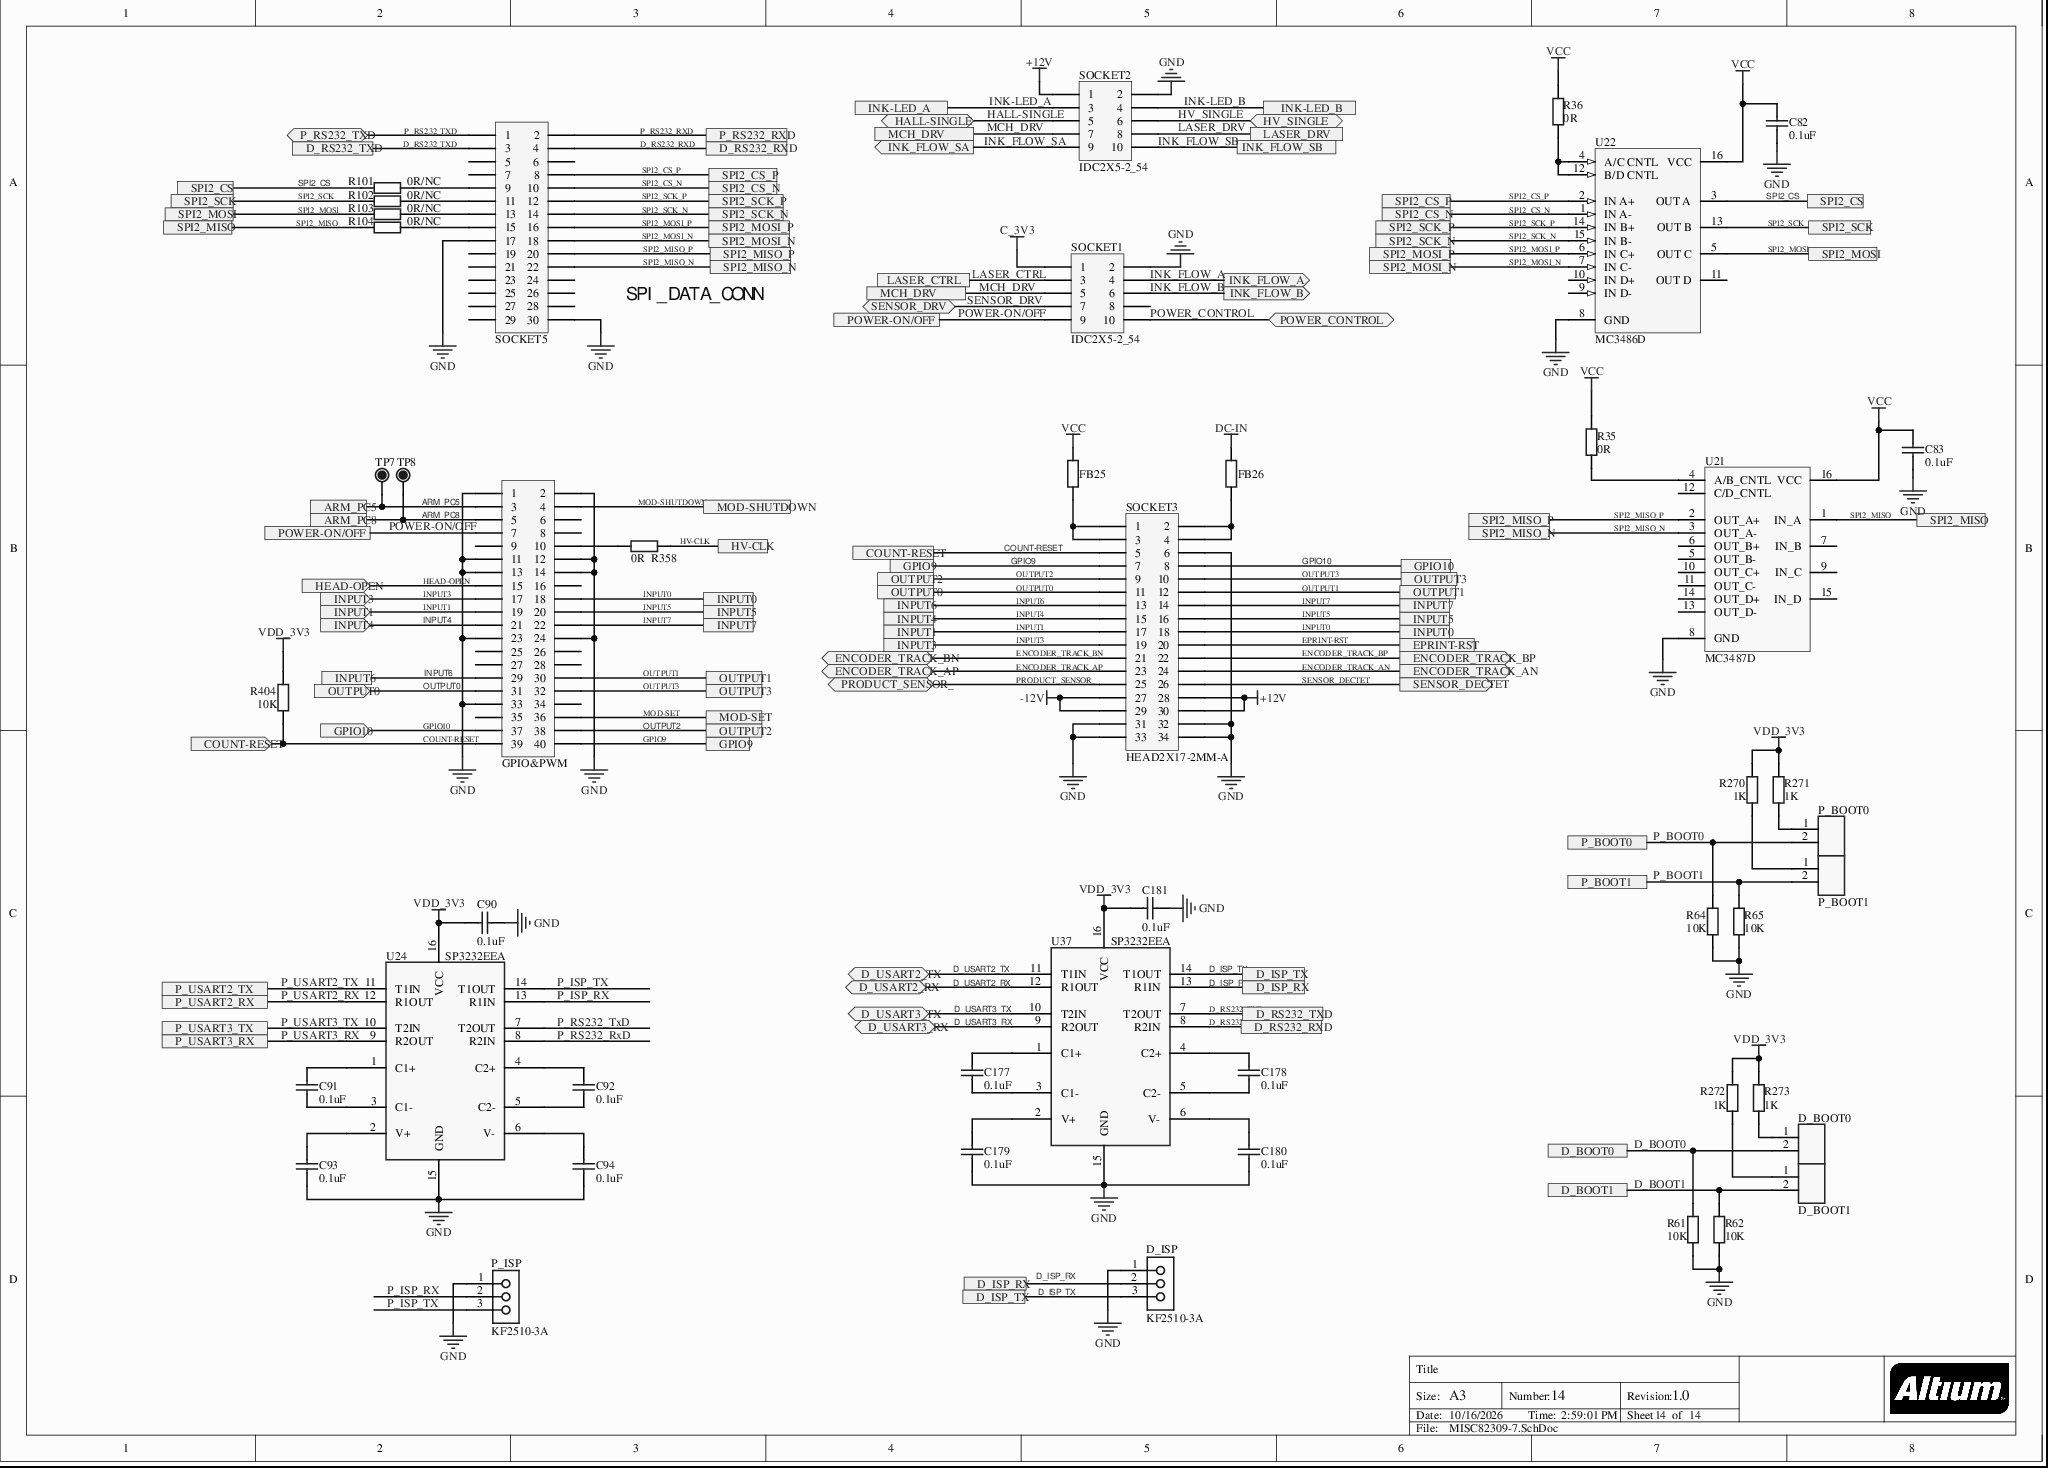
[diagram p0: MISC82309-7.SchDoc]
# Altium project MISC82309-16.PrjPcb (part 6 of 6)

## Sheet MISC82309-7.SchDoc
size A3; DocumentNumber: 14; Revision: 1.0; SheetNumber: 14; SheetTotal: 14

### Parts
C82  0.1uF  [CAP_0805]
C83  0.1uF  [CAP_0805]
C90  0.1uF  [C0603]
C91  0.1uF  [C0603]
C92  0.1uF  [C0603]
C93  0.1uF  [C0603]
C94  0.1uF  [C0603]
C177  0.1uF  [C0603]
C178  0.1uF  [C0603]
C179  0.1uF  [C0603]
C180  0.1uF  [C0603]
C181  0.1uF  [C0603]
D_BOOT0  PLS-2  [PLS-2-2_54]  (value not drawn)
D_BOOT1  PLS-2  [PLS-2-2_54]  (value not drawn)
D_ISP  KF2510-3A  [KF2510-3A]
FB25  60  [SMD1206-L]  (value not drawn)
FB26  60  [SMD1206-L]  (value not drawn)
GPIO&PWM  HEAD2X20-2MM-A  [IDC2X20-2.0mm-A]  (value not drawn)
P_BOOT0  PLS-2  [PLS-2-2_54]  (value not drawn)
P_BOOT1  PLS-2  [PLS-2-2_54]  (value not drawn)
P_ISP  KF2510-3A  [KF2510-3A]
R35  0R  [RES_0603]
R36  0R  [RES_0603]
R61  10K  [RES_0603]
R62  10K  [RES_0603]
R64  10K  [RES_0603]
R65  10K  [RES_0603]
R101  0R/NC  [RES_0603]
R102  0R/NC  [RES_0603]
R103  0R/NC  [RES_0603]
R104  0R/NC  [RES_0603]
R270  1K  [RES_0603]
R271  1K  [RES_0603]
R272  1K  [RES_0603]
R273  1K  [RES_0603]
R358  0R  [RES_0603]
R404  10K  [RES_0603]
SOCKET1  IDC2X5-2_54  [IDC2X5-2_54]
SOCKET2  IDC2X5-2_54  [IDC2X5-2_54]
SOCKET3  HEAD2X17-2MM-A  [IDC2X17-2.0mm-A]
SOCKET5  HEAD2X15-2MM-A  [IDC2X15-2.0mm-A]  (value not drawn)
TP7  TP  [TPOINT]  (value not drawn)
TP8  TP  [TPOINT]  (value not drawn)
U21  MC3487D  [751B-03_N]
U22  MC3486D  [751B-03_N]
U24  SP3232EEA  [SSOP16_M]
U37  SP3232EEA  [SSOP16_M]

### Ports
ARM_PC5, ARM_PC8, COUNT-RESET, COUNT-RESET (in), D_BOOT0, D_BOOT1, D_ISP_RX, D_ISP_TX, D_RS232_RXD, D_RS232_TXD, D_USART2_RX (bidir), D_USART2_TX (bidir), D_USART3_RX (bidir), D_USART3_TX (bidir), ENCODER_TRACK_AN (out), ENCODER_TRACK_AP (bidir), ENCODER_TRACK_BN (bidir), ENCODER_TRACK_BP (out), EPRINT-RST, GPIO9, GPIO10, GPIO10 (in), HALL-SINGLE (bidir), HEAD-OPEN (in), HV-CLK, HV_SINGLE (bidir), INK-LED_A, INK-LED_B, INK_FLOW_A (out), INK_FLOW_B (out), INK_FLOW_SA (out), INK_FLOW_SB, INPUT0, INPUT1, INPUT1 (in), INPUT3, INPUT3 (in), INPUT4, INPUT4 (in), INPUT5, INPUT6, INPUT7, LASER_CTRL, LASER_DRV, MCH_DRV, MOD-SET, MOD-SHUTDOWN, OUTPUT0, OUTPUT0 (in), OUTPUT1, OUTPUT2, OUTPUT3, P_BOOT0, P_BOOT1, P_RS232_RXD, P_RS232_TXD (bidir), P_USART2_RX, P_USART2_TX, P_USART3_RX, P_USART3_TX, POWER-ON/OFF, POWER_CONTROL (bidir), PRODUCT_SENSOR_ (bidir), SENSOR_DECTET (out), SENSOR_DRV (bidir), SPI2_CS, SPI2_CS_N, SPI2_CS_P, SPI2_MISO, SPI2_MISO_N, SPI2_MISO_P, SPI2_MOSI, SPI2_MOSI_N, SPI2_MOSI_P, SPI2_SCK, SPI2_SCK_N, SPI2_SCK_P

### Nets
+12V: SOCKET2.1 SOCKET3.28 SOCKET3.30
-12V: SOCKET3.27 SOCKET3.29
C_3V3: SOCKET1.1
DC-IN: FB26.1
GND: C82.1 C83.1 C90.1 C93.1 C94.1 C179.1 C180.1 C181.1 D_ISP.1 GPIO&PWM.1 GPIO&PWM.2 GPIO&PWM.11 GPIO&PWM.12 GPIO&PWM.13 GPIO&PWM.14 GPIO&PWM.23 GPIO&PWM.24 GPIO&PWM.33 P_ISP.1 R61.2 R62.2 R64.2 R65.2 SOCKET1.2 SOCKET2.2 SOCKET3.6 SOCKET3.31 SOCKET3.32 SOCKET3.33 SOCKET3.34 SOCKET5.17 SOCKET5.30 U21.8(GND) U22.8(GND) U24.15(GND) U37.15(GND)
VCC: C82.2 C83.2 FB25.1 R35.2 R36.2 U21.16(VCC) U22.16(VCC)
VDD_3V3: C90.2 C181.2 R270.2 R271.2 R272.2 R273.2 R404.1 U24.16(VCC) U37.16(VCC)
ARM_PC5: GPIO&PWM.3 TP7.1 ; port ARM_PC5
ARM_PC8: GPIO&PWM.5 TP8.1 ; port ARM_PC8
COUNT-RESET: GPIO&PWM.39 R404.2 SOCKET3.5 ; port COUNT-RESET
D_BOOT0: D_BOOT0.2 R61.1 ; port D_BOOT0
D_BOOT1: D_BOOT1.2 R62.1 ; port D_BOOT1
D_ISP_RX: D_ISP.2 U37.13(R1IN) ; port D_ISP_RX
D_ISP_TX: D_ISP.3 U37.14(T1OUT) ; port D_ISP_TX
D_RS232_RXD: SOCKET5.4 U37.8(R2IN) ; port D_RS232_RXD
D_RS232_TXD: SOCKET5.3 U37.7(T2OUT) ; port D_RS232_TXD
D_USART2_RX: U37.12(R1OUT) ; port D_USART2_RX
D_USART2_TX: U37.11(T1IN) ; port D_USART2_TX
D_USART3_RX: U37.9(R2OUT) ; port D_USART3_RX
D_USART3_TX: U37.10(T2IN) ; port D_USART3_TX
ENCODER_TRACK_AN: SOCKET3.24 ; port ENCODER_TRACK_AN
ENCODER_TRACK_AP: SOCKET3.23 ; port ENCODER_TRACK_AP
ENCODER_TRACK_BN: SOCKET3.21 ; port ENCODER_TRACK_BN
ENCODER_TRACK_BP: SOCKET3.22 ; port ENCODER_TRACK_BP
EPRINT-RST: SOCKET3.20 ; port EPRINT-RST
GPIO9: GPIO&PWM.40 SOCKET3.7 ; port GPIO9
GPIO10: GPIO&PWM.37 SOCKET3.8 ; port GPIO10
HALL-SINGLE: SOCKET2.5 ; port HALL-SINGLE
HEAD-OPEN: GPIO&PWM.15 ; port HEAD-OPEN
HV-CLK: R358.2 ; port HV-CLK
HV_SINGLE: SOCKET2.6 ; port HV_SINGLE
INK-LED_A: SOCKET2.3 ; port INK-LED_A
INK-LED_B: SOCKET2.4 ; port INK-LED_B
INK_FLOW_A: SOCKET1.4 ; port INK_FLOW_A
INK_FLOW_B: SOCKET1.6 ; port INK_FLOW_B
INK_FLOW_SA: SOCKET2.9 ; port INK_FLOW_SA
INK_FLOW_SB: SOCKET2.10 ; port INK_FLOW_SB
INPUT0: GPIO&PWM.18 SOCKET3.18 ; port INPUT0
INPUT1: GPIO&PWM.19 SOCKET3.17 ; port INPUT1
INPUT3: GPIO&PWM.17 SOCKET3.19 ; port INPUT3
INPUT4: GPIO&PWM.21 SOCKET3.15 ; port INPUT4
INPUT5: GPIO&PWM.20 SOCKET3.16 ; port INPUT5
INPUT6: GPIO&PWM.29 SOCKET3.13 ; port INPUT6
INPUT7: GPIO&PWM.22 SOCKET3.14 ; port INPUT7
LASER_CTRL: SOCKET1.3 ; port LASER_CTRL
LASER_DRV: SOCKET2.8 ; port LASER_DRV
MCH_DRV: SOCKET1.5 SOCKET2.7 ; port MCH_DRV
MOD-SET: GPIO&PWM.36 ; port MOD-SET
MOD-SHUTDOWN: GPIO&PWM.4 ; port MOD-SHUTDOWN
OUTPUT0: GPIO&PWM.31 SOCKET3.11 ; port OUTPUT0
OUTPUT1: GPIO&PWM.30 SOCKET3.12 ; port OUTPUT1
OUTPUT2: GPIO&PWM.38 SOCKET3.9 ; port OUTPUT2
OUTPUT3: GPIO&PWM.32 SOCKET3.10 ; port OUTPUT3
P_BOOT0: P_BOOT0.2 R64.1 ; port P_BOOT0
P_BOOT1: P_BOOT1.2 R65.1 ; port P_BOOT1
P_ISP_RX: P_ISP.2 U24.13(R1IN)
P_ISP_TX: P_ISP.3 U24.14(T1OUT)
P_RS232_RXD: SOCKET5.2 U24.8(R2IN) ; port P_RS232_RXD
P_RS232_TXD: SOCKET5.1 U24.7(T2OUT) ; port P_RS232_TXD
P_USART2_RX: U24.12(R1OUT) ; port P_USART2_RX
P_USART2_TX: U24.11(T1IN) ; port P_USART2_TX
P_USART3_RX: U24.9(R2OUT) ; port P_USART3_RX
P_USART3_TX: U24.10(T2IN) ; port P_USART3_TX
POWER-ON/OFF: GPIO&PWM.7 SOCKET1.9 ; port POWER-ON/OFF
POWER_CONTROL: SOCKET1.10 ; port POWER_CONTROL
PRODUCT_SENSOR_: SOCKET3.25 ; port PRODUCT_SENSOR_
SENSOR_DECTET: SOCKET3.26 ; port SENSOR_DECTET
SENSOR_DRV: SOCKET1.7 ; port SENSOR_DRV
SPI2_CS: R101.1 U22.3(OUT_A) ; port SPI2_CS
SPI2_CS_N: SOCKET5.10 U22.1(IN_A-) ; port SPI2_CS_N
SPI2_CS_P: SOCKET5.8 U22.2(IN_A+) ; port SPI2_CS_P
SPI2_MISO: R104.1 U21.1(IN_A) ; port SPI2_MISO  [project net P_JNTRST]
SPI2_MISO_N: SOCKET5.22 U21.3(OUT_A-) ; port SPI2_MISO_N
SPI2_MISO_P: SOCKET5.20 U21.2(OUT_A+) ; port SPI2_MISO_P
SPI2_MOSI: R103.1 U22.5(OUT_C) ; port SPI2_MOSI
SPI2_MOSI_N: SOCKET5.18 U22.7(IN_C-) ; port SPI2_MOSI_N
SPI2_MOSI_P: SOCKET5.16 U22.6(IN_C+) ; port SPI2_MOSI_P
SPI2_SCK: R102.1 U22.13(OUT_B) ; port SPI2_SCK  [project net P_JTDO]
SPI2_SCK_N: SOCKET5.14 U22.15(IN_B-) ; port SPI2_SCK_N
SPI2_SCK_P: SOCKET5.12 U22.14(IN_B+) ; port SPI2_SCK_P
NetC91_1: C91.1 U24.3(C1-)
NetC91_2: C91.2 U24.1(C1+)
NetC92_1: C92.1 U24.5(C2-)
NetC92_2: C92.2 U24.4(C2+)
NetC93_2: C93.2 U24.2(V+)
NetC94_2: C94.2 U24.6(V-)
NetC177_1: C177.1 U37.3(C1-)
NetC177_2: C177.2 U37.1(C1+)
NetC178_1: C178.1 U37.5(C2-)
NetC178_2: C178.2 U37.4(C2+)
NetC179_2: C179.2 U37.2(V+)
NetC180_2: C180.2 U37.6(V-)
NetD_BOOT0_1: D_BOOT0.1 R273.1
NetD_BOOT1_1: D_BOOT1.1 R272.1
NetFB25_2: FB25.2 SOCKET3.1 SOCKET3.3
NetFB26_2: FB26.2 SOCKET3.2 SOCKET3.4
NetGPIO&PWM_10: GPIO&PWM.10 R358.1
NetP_BOOT0_1: P_BOOT0.1 R271.1
NetP_BOOT1_1: P_BOOT1.1 R270.1
NetR35_1: R35.1 U21.4(A/B_CNTL)
NetR36_1: R36.1 U22.4(A/C_CNTL) U22.12(B/D_CNTL)
NetR101_2: R101.2 SOCKET5.9
NetR102_2: R102.2 SOCKET5.11
NetR103_2: R103.2 SOCKET5.13
NetR104_2: R104.2 SOCKET5.15

Not connected (* = marked no-connect by the designer): GPIO&PWM 6 8 9 16 25 26 27 28 34 35; SOCKET1 8; SOCKET5 5 6 7 19 21 23 24 25 26 27 28 29; U21 5(OUT_B-) 6(OUT_B+) 7(IN_B) 9(IN_C) 10(OUT_C+) 11(OUT_C-) 12(C/D_CNTL) 13(OUT_D-) 14(OUT_D+) 15(IN_D); U22 9(IN_D-)* 10(IN_D+)* 11(OUT_D)

### Notes on the sheet
- SPI_DATA_CONN
- Labels drawn without touching a wire or pin: D_ISP_RX
- Title
- Size:
- Date:
- A3
- Number:
- Time:
- Revision:
- Sheet
- of
- File:

### Library data of the parts
C82 C83 = CAP_0805: Capacitor; value: 0.1uF
C90-C94 C177-C181 = CAP_0402: Capacitor; value: 0.1uF
FB25 FB26 = FB: Res; value: 10K
R35 R36 R61 R62 R64 R65 R101-R104 R270-R273 R358 R404 = Res_0603: Res
  R35 R36 R358: value: 0R
  R61 R62 R64 R65 R404: value: 10K
  R101-R104: value: 0R/NC
  R270-R273: value: 1K
SOCKET1 SOCKET2 = HEAD2X5-2_54
TP7 TP8 = TP: Test Point; OriginalSymbolOrigin: (0,0)
U21 = MC3487D: Quad EIA-422/423 Line Receiver; Published: 17-Jul-2002; LatestRevisionDate: 13-Apr-2006; LatestRevisionNote: IPC-7351 Footprint Added.; DatasheetVersion: 1988; PackageVersion: 1991; PackageReference: 751B-03; PackageDescription: 16-Pin Small Outline Integrated Circuit 1.27 mm Pitch; Code_JEDEC: MS-012-AC; Code_IPC: SOIC127P600-16; ComponentLink1Description: Manufacturer Link; ComponentLink1URL: http://www.onsemi.com/site/products/parametrics/0,4446,178,00.html; PCB DECAL: 751B-03_N; Comment_1: MC3487D; Publisher: Altium Limited
U22 = MC3486D: Quad EIA-422/423 Line Receiver; Published: 17-Jul-2002; LatestRevisionDate: 13-Apr-2006; LatestRevisionNote: IPC-7351 Footprint Added.; DatasheetVersion: 1988; PackageVersion: 1991; PackageReference: 751B-03; PackageDescription: 16-Pin Small Outline Integrated Circuit 1.27 mm Pitch; Code_JEDEC: MS-012-AC; Code_IPC: SOIC127P600-16; ComponentLink1Description: Manufacturer Link; ComponentLink1URL: http://www.onsemi.com/site/products/parametrics/0,4446,178,00.html; Publisher: Altium Limited
U24 U37 = MAX3232

## Nets that join several sheets
+12V: MISC82309-15 (6 pins), MISC82309-12 (C57.1 C63.2 D15.1 U15.3), MISC82309-5 (C155.1 C158.1 FB5.1), MISC82309-3 (C171.1 C172.2 FB19.1), MISC82309-9 (5 pins), MISC82309-7 (SOCKET2.1 SOCKET3.28 SOCKET3.30)
+18V: MISC82309-15 (C153.1 D10.1 U62.3), MISC82309-12 (C50.1 C52.1 U13.8 U14.7), MISC82309-5 (C28.1 U7.7), MISC82309-6 (C267.1 U23.7)
-12V: MISC82309-15 (9 pins), MISC82309-12 (C64.2 C65.2 FB3.1), MISC82309-5 (8 pins), MISC82309-6 (5 pins), MISC82309-3 (C174.2 C175.2 FB20.1), MISC82309-7 (SOCKET3.27 SOCKET3.29)
-VCC: MISC82309-3 (U61.6), MISC82309-4 (C423.1 C424.2 U63.6 U65.1)
C_3V3: MISC82309-15 (6 pins), MISC82309-8 (26 pins), MISC82309-7 (SOCKET1.1)
DAC_+12V: MISC82309-5 (C89.2 FB5.2 U107.8), MISC82309-6 (U48.8)
DAC_-12V: MISC82309-5 (C79.2 FB6.2 U107.4), MISC82309-6 (U48.4)
DC-IN: MISC82309-15 (17 pins), MISC82309-12 (5 pins), MISC82309-5 (5 pins), MISC82309-6 (5 pins), MISC82309-9 (C230.2 C231.2 U46.7 U46.8), MISC82309-7 (FB26.1)
DET+12V: MISC82309-3 (R204.2 Radj6.3 U36.4), MISC82309-4 (Radj12.3 U51.4)
DET-12V: MISC82309-3 (R205.2 U36.11), MISC82309-4 (U51.11)
GND: MISC82309-15 (53 pins), MISC82309-11 (54 pins), MISC82309-10 (41 pins), MISC82309-8 (25 pins), MISC82309-13 (C147.1 C148.1 U9.12 U9.34), MISC82309-12 (37 pins), MISC82309-5 (38 pins), MISC82309-6 (32 pins), MISC82309-3 (40 pins), MISC82309-4 (22 pins), MISC82309-14 (28 pins), MISC82309-9 (23 pins), MISC82309-7 (36 pins)
VCC: MISC82309-15 (14 pins), MISC82309-11 (Q8.2 R150.2), MISC82309-12 (C56.1 U15.11 U49.14 U52.1), MISC82309-3 (U61.3), MISC82309-4 (R479.2 U63.3), MISC82309-14 (10 pins), MISC82309-9 (U40.8 U49.14), MISC82309-7 (7 pins)
VDD_3V3: MISC82309-15 (6 pins), MISC82309-11 (41 pins), MISC82309-10 (34 pins), MISC82309-13 (C147.2 C148.2 U9.11 U9.33), MISC82309-12 (U52.23 U52.24), MISC82309-5 (C30.1 C31.1 U109.24 U109.27), MISC82309-6 (C282.1 C283.1 U110.24 U110.27), MISC82309-3 (6 pins), MISC82309-14 (C220.2 Q25.3 R283.2), MISC82309-7 (9 pins)
ARM_PC5: MISC82309-11 (U10.45), MISC82309-7 (GPIO&PWM.3 TP7.1)
ARM_PC8: MISC82309-11 (U10.7), MISC82309-7 (GPIO&PWM.5 TP8.1)
CH-DET_A: MISC82309-10 (R207.1), MISC82309-3 (R199.2 U36.7)
CH-DET_B: MISC82309-10 (R110.1), MISC82309-4 (R339.2 U51.7)
CH_A: MISC82309-10 (U17.1), MISC82309-3 (R378.2)
CH_B: MISC82309-10 (U17.2), MISC82309-4 (R379.2)
CH_PHASE1: MISC82309-10 (U17.15), MISC82309-8 (U16.17)
CH_PHASE2: MISC82309-10 (U17.16), MISC82309-8 (U16.18)
CH_PHASE3: MISC82309-10 (U17.17), MISC82309-8 (U16.19)
CH_PHASE4: MISC82309-10 (U17.18), MISC82309-8 (U16.20)
CH_PHASE5: MISC82309-10 (U17.33), MISC82309-8 (U16.21)
CH_PHASE6: MISC82309-10 (U17.34), MISC82309-8 (U16.26)
CH_PHASE7: MISC82309-10 (U17.63), MISC82309-8 (U16.27)
CH_PHASE8: MISC82309-10 (U17.64), MISC82309-8 (U16.28)
CHARGE-CTRL_A: MISC82309-11 (U10.20), MISC82309-5 (R151.2 R312.2)
CHARGE-CTRL_B: MISC82309-11 (U10.21), MISC82309-6 (R343.2 R344.2)
COUNT-RESET: MISC82309-11 (U10.35), MISC82309-7 (GPIO&PWM.39 R404.2 SOCKET3.5)
D_A0: MISC82309-13 (R547.1), MISC82309-5 (U109.12)
D_A1: MISC82309-13 (R548.1), MISC82309-5 (U109.11)
D_A2: MISC82309-13 (R549.1), MISC82309-5 (U109.10)
D_A3: MISC82309-13 (R550.1), MISC82309-5 (U109.9)
D_A4: MISC82309-13 (R525.1), MISC82309-5 (U109.8)
D_A5: MISC82309-13 (R526.1), MISC82309-5 (U109.7)
D_A6: MISC82309-13 (R527.1), MISC82309-5 (U109.6)
D_A7: MISC82309-13 (R528.1), MISC82309-5 (U109.5)
D_A8: MISC82309-13 (R529.1), MISC82309-5 (U109.4)
D_A9: MISC82309-13 (R530.1), MISC82309-5 (U109.3)
D_A10: MISC82309-13 (R531.1), MISC82309-5 (U109.2)
D_A11: MISC82309-13 (R532.1), MISC82309-5 (U109.1)
D_B0: MISC82309-13 (R533.1), MISC82309-6 (U110.12)
D_B1: MISC82309-13 (R534.1), MISC82309-6 (U110.11)
D_B2: MISC82309-13 (R535.1), MISC82309-6 (U110.10)
D_B3: MISC82309-13 (R536.1), MISC82309-6 (U110.9)
D_B4: MISC82309-13 (R537.1), MISC82309-6 (U110.8)
D_B5: MISC82309-13 (R538.1), MISC82309-6 (U110.7)
D_B6: MISC82309-13 (R539.1), MISC82309-6 (U110.6)
D_B7: MISC82309-13 (R540.1), MISC82309-6 (U110.5)
D_B8: MISC82309-13 (R541.1), MISC82309-6 (U110.4)
D_B9: MISC82309-13 (R542.1), MISC82309-6 (U110.3)
D_B10: MISC82309-13 (R543.1), MISC82309-6 (U110.2)
D_B11: MISC82309-13 (R544.1), MISC82309-6 (U110.1)
D_BOOT0: MISC82309-10 (U17.94), MISC82309-7 (D_BOOT0.2 R61.1)
D_BOOT1: MISC82309-10 (U17.37), MISC82309-7 (D_BOOT1.2 R62.1)
D_OUT: MISC82309-11 (U10.41), MISC82309-8 (R558.1)
D_USART2_RX: MISC82309-10 (U17.87), MISC82309-7 (U37.12)
D_USART2_TX: MISC82309-10 (U17.86), MISC82309-7 (U37.11)
D_USART3_RX: MISC82309-10 (U17.48), MISC82309-7 (U37.9)
D_USART3_TX: MISC82309-10 (U17.47), MISC82309-7 (U37.10)
DAC_CLK_A: MISC82309-8 (U16.52), MISC82309-5 (U109.28)
DAC_CLK_B: MISC82309-8 (U16.53), MISC82309-6 (U110.28)
DET_D0: MISC82309-10 (U17.61), MISC82309-3 (U64.37)
DET_D1: MISC82309-10 (U17.62), MISC82309-3 (U64.38)
DET_D2: MISC82309-10 (U17.81), MISC82309-3 (U64.39)
DET_D3: MISC82309-10 (U17.82), MISC82309-3 (U64.40)
DET_D4: MISC82309-10 (U17.38), MISC82309-3 (U64.41)
DET_D5: MISC82309-10 (U17.39), MISC82309-3 (U64.42)
DET_D6: MISC82309-10 (U17.40), MISC82309-3 (U64.43)
DET_D7: MISC82309-10 (U17.41), MISC82309-3 (U64.44)
DET_D8: MISC82309-10 (U17.42), MISC82309-3 (U64.24)
DET_D9: MISC82309-10 (U17.43), MISC82309-3 (U64.23)
DET_D10: MISC82309-10 (U17.44), MISC82309-3 (U64.22)
DET_D11: MISC82309-10 (U17.45), MISC82309-3 (U64.21)
DET_D12: MISC82309-10 (U17.46), MISC82309-3 (U64.20)
DET_D13: MISC82309-10 (U17.55), MISC82309-3 (U64.19)
DET_D14: MISC82309-10 (U17.56), MISC82309-3 (U64.18)
DET_D15: MISC82309-10 (U17.57), MISC82309-3 (U64.17)
DETECT-RST: MISC82309-10 (U17.95), MISC82309-8 (U16.86)
DROP-CH_A: MISC82309-10 (R206.1), MISC82309-3 (R556.1)
DROP-CH_B: MISC82309-10 (R106.1), MISC82309-4 (R578.1 Radj11.2)
DROP_A: MISC82309-11 (U10.27), MISC82309-8 (U16.73)
DROP_B: MISC82309-11 (U10.28), MISC82309-8 (U16.75)
ENC_A: MISC82309-10 (R518.2), MISC82309-8 (R409.2), MISC82309-3 (U64.47)
ENC_B: MISC82309-10 (R519.2), MISC82309-8 (R410.2), MISC82309-3 (U64.14)
ENCODE_PA: MISC82309-11 (R567.2 U10.42), MISC82309-14 (U31.5)
ENCODE_PB: MISC82309-11 (R569.2 U10.43), MISC82309-14 (U31.3)
ENCODER_TRACK_AN: MISC82309-14 (U31.7), MISC82309-7 (SOCKET3.24)
ENCODER_TRACK_AP: MISC82309-14 (U31.6), MISC82309-7 (SOCKET3.23)
ENCODER_TRACK_BN: MISC82309-14 (U31.1), MISC82309-7 (SOCKET3.21)
ENCODER_TRACK_BP: MISC82309-14 (U31.2), MISC82309-7 (SOCKET3.22)
EPRINT-RST: MISC82309-11 (U10.126), MISC82309-7 (SOCKET3.20)
FSMC_A0: MISC82309-11 (U10.10), MISC82309-13 (U9.1)
FSMC_A1: MISC82309-11 (U10.11), MISC82309-13 (U9.2)
FSMC_A2: MISC82309-11 (U10.12), MISC82309-13 (U9.3)
FSMC_A3: MISC82309-11 (U10.13), MISC82309-13 (U9.4)
FSMC_A4: MISC82309-11 (U10.14), MISC82309-13 (U9.5)
FSMC_A5: MISC82309-11 (U10.15), MISC82309-13 (U9.18)
FSMC_A6: MISC82309-11 (U10.50), MISC82309-13 (U9.19)
FSMC_A7: MISC82309-11 (U10.53), MISC82309-13 (U9.20)
FSMC_A8: MISC82309-11 (U10.54), MISC82309-13 (U9.21)
FSMC_A9: MISC82309-11 (U10.55), MISC82309-13 (U9.22)
FSMC_A10: MISC82309-11 (U10.56), MISC82309-13 (U9.23)
FSMC_A11: MISC82309-11 (U10.57), MISC82309-13 (U9.24)
FSMC_A12: MISC82309-11 (U10.87), MISC82309-13 (U9.25)
FSMC_A13: MISC82309-11 (U10.88), MISC82309-13 (U9.26)
FSMC_A14: MISC82309-11 (U10.89), MISC82309-13 (U9.27)
FSMC_A15: MISC82309-11 (U10.90), MISC82309-13 (U9.42)
FSMC_A16: MISC82309-11 (U10.80), MISC82309-13 (U9.43)
FSMC_A17: MISC82309-11 (U10.81), MISC82309-13 (U9.44)
FSMC_A18: MISC82309-11 (U10.82), MISC82309-13 (U9.28)
FSMC_D0: MISC82309-11 (U10.85), MISC82309-13 (R533.2 R547.2 U9.7)
FSMC_D1: MISC82309-11 (U10.86), MISC82309-13 (R534.2 R548.2 U9.8)
FSMC_D2: MISC82309-11 (U10.114), MISC82309-13 (R535.2 R549.2 U9.9)
FSMC_D3: MISC82309-11 (U10.115), MISC82309-13 (R536.2 R550.2 U9.10)
FSMC_D4: MISC82309-11 (U10.58), MISC82309-13 (R525.2 R537.2 U9.13)
FSMC_D5: MISC82309-11 (U10.59), MISC82309-13 (R526.2 R538.2 U9.14)
FSMC_D6: MISC82309-11 (U10.60), MISC82309-13 (R527.2 R539.2 U9.15)
FSMC_D7: MISC82309-11 (U10.63), MISC82309-13 (R528.2 R540.2 U9.16)
FSMC_D8: MISC82309-11 (U10.64), MISC82309-13 (R529.2 R541.2 U9.29)
FSMC_D9: MISC82309-11 (U10.65), MISC82309-13 (R530.2 R542.2 U9.30)
FSMC_D10: MISC82309-11 (U10.66), MISC82309-13 (R531.2 R543.2 U9.31)
FSMC_D11: MISC82309-11 (U10.67), MISC82309-13 (R532.2 R544.2 U9.32)
FSMC_D12: MISC82309-11 (U10.68), MISC82309-13 (U9.35)
FSMC_D13: MISC82309-11 (U10.77), MISC82309-13 (U9.36)
FSMC_D14: MISC82309-11 (U10.78), MISC82309-13 (U9.37)
FSMC_D15: MISC82309-11 (U10.79), MISC82309-13 (U9.38)
FSMC_NBL0: MISC82309-11 (U10.141), MISC82309-13 (U9.39)
FSMC_NBL1: MISC82309-11 (U10.142), MISC82309-13 (U9.40)
FSMC_NE1: MISC82309-11 (U10.123), MISC82309-13 (U9.6)
FSMC_NE2: MISC82309-11 (U10.124), MISC82309-8 (U16.55)
FSMC_NE3: MISC82309-11 (U10.125), MISC82309-8 (U16.56)
FSMC_NOE: MISC82309-11 (U10.118), MISC82309-13 (U9.41)
FSMC_NWE: MISC82309-11 (U10.119), MISC82309-8 (U16.54), MISC82309-13 (U9.17)
HALL-SINGLE: MISC82309-14 (R491.1), MISC82309-7 (SOCKET2.5)
HALL-SWITCH: MISC82309-11 (U10.29), MISC82309-14 (U32.4)
HEAD-OPEN: MISC82309-8 (U16.70), MISC82309-7 (GPIO&PWM.15)
HV-CLK: MISC82309-11 (R391.2), MISC82309-8 (R347.2), MISC82309-12 (U52.18), MISC82309-7 (R358.2)
HV-CONTROL: MISC82309-11 (U10.112), MISC82309-12 (U52.17)
HV-SHUTDOWN: MISC82309-12 (U52.7), MISC82309-9 (U45.2)
HV_CLK: MISC82309-12 (U52.6), MISC82309-9 (U49.9)
HV_PWM: MISC82309-12 (U52.5), MISC82309-9 (R285.1 R286.2)
HV_S: MISC82309-11 (U10.26), MISC82309-14 (U32.6)
HV_SENSOR: MISC82309-11 (U10.34), MISC82309-9 (D33.2)
HV_SET: MISC82309-11 (R392.2), MISC82309-12 (U52.19)
HV_SINGLE: MISC82309-14 (R166.1), MISC82309-7 (SOCKET2.6)
INK-LED_A: MISC82309-14 (R212.2), MISC82309-7 (SOCKET2.3)
INK-LED_B: MISC82309-14 (R386.2), MISC82309-7 (SOCKET2.4)
INK_DETECTING: MISC82309-11 (U10.98), MISC82309-10 (U17.98)
INK_FLOW_A: MISC82309-14 (D31.2), MISC82309-7 (SOCKET1.4)
INK_FLOW_B: MISC82309-14 (D131.2), MISC82309-7 (SOCKET1.6)
INK_FLOW_SA: MISC82309-14 (R172.2 R173.2), MISC82309-7 (SOCKET2.9)
INK_FLOW_SB: MISC82309-14 (R372.2 R373.2), MISC82309-7 (SOCKET2.10)
INK_PRINTING: MISC82309-11 (U10.100), MISC82309-10 (U17.97)
LASER_CTRL: MISC82309-14 (Q26.1), MISC82309-7 (SOCKET1.3)
LASER_DRV: MISC82309-14 (C221.2 D40.2 Q25.2), MISC82309-7 (SOCKET2.8)
MOD-CLK: MISC82309-8 (U16.66), MISC82309-12 (U49.1)
MOD-CONTROL: MISC82309-11 (U10.116), MISC82309-12 (U52.20)
MOD-LED_A: MISC82309-8 (U16.67), MISC82309-14 (U32.9)
MOD-LED_B: MISC82309-8 (U16.68), MISC82309-14 (U49.13)
MOD-SET: MISC82309-11 (R508.2), MISC82309-12 (U52.21), MISC82309-7 (GPIO&PWM.36)
MOD-SHUTDOWN: MISC82309-12 (U15.13 U52.4), MISC82309-7 (GPIO&PWM.4)
MOD_CTRL: MISC82309-11 (U10.122), MISC82309-12 (R67.2 R68.2)
OE_A: MISC82309-11 (R509.1), MISC82309-8 (U16.72)
OE_B: MISC82309-11 (R511.1), MISC82309-8 (U16.74)
OUT+: MISC82309-3 (R419.1), MISC82309-4 (C501.1 R523.1 U63.4)
OUT-: MISC82309-3 (R418.2), MISC82309-4 (C502.1 R524.1 U63.5)
P_BOOT0: MISC82309-11 (U10.138), MISC82309-7 (P_BOOT0.2 R64.1)
P_BOOT1: MISC82309-11 (U10.48), MISC82309-7 (P_BOOT1.2 R65.1)
P_JNTRST: MISC82309-11 (P-JTAG.3 R407.2 R589.1 U10.134), MISC82309-7 (R104.1 U21.1)
P_JTDO: MISC82309-11 (P-JTAG.6 R406.2 R590.1 U10.133), MISC82309-7 (R102.1 U22.13)
P_USART2_RX: MISC82309-11 (U10.37), MISC82309-7 (U24.12)
P_USART2_TX: MISC82309-11 (U10.36), MISC82309-7 (U24.11)
P_USART3_RX: MISC82309-11 (U10.70), MISC82309-7 (U24.9)
P_USART3_TX: MISC82309-11 (U10.69), MISC82309-7 (U24.10)
POWER_CONTROL: MISC82309-15 (R8.1), MISC82309-7 (SOCKET1.10)
PRE-CH_A: MISC82309-11 (R349.2), MISC82309-10 (R515.2 R565.1), MISC82309-8 (R345.2), MISC82309-14 (U32.13)
PRE-CH_B: MISC82309-11 (R348.2), MISC82309-10 (R516.2 R564.1), MISC82309-8 (R346.2), MISC82309-14 (U32.11)
PRE-CHARGE_A: MISC82309-5 (Radj2.1), MISC82309-14 (U32.12)
PRE-CHARGE_B: MISC82309-6 (Radj9.1), MISC82309-14 (U32.10)
PRINT-RST: MISC82309-11 (U10.93), MISC82309-8 (U16.85)
PRODUCT-S: MISC82309-11 (U10.44), MISC82309-14 (U32.2)
PRODUCT_SENSOR_: MISC82309-14 (R493.1), MISC82309-7 (SOCKET3.25)
SENSOR_DECTET: MISC82309-14 (R155.1), MISC82309-7 (SOCKET3.26)
SENSOR_DRV: MISC82309-14 (C163.2 C363.2 R175.1 R375.1), MISC82309-7 (SOCKET1.7)
SPI2_CS: MISC82309-11 (R405.2 U10.40), MISC82309-7 (R101.1 U22.3)
SPI2_MOSI: MISC82309-11 (R408.2 U10.135), MISC82309-7 (R103.1 U22.5)
USART6_RX: MISC82309-11 (U10.97), MISC82309-10 (R513.2)
USART6_TX: MISC82309-11 (U10.96), MISC82309-10 (R514.2)
VOCM: MISC82309-3 (C599.1 R598.1 R599.2 U61.2), MISC82309-4 (U63.2)